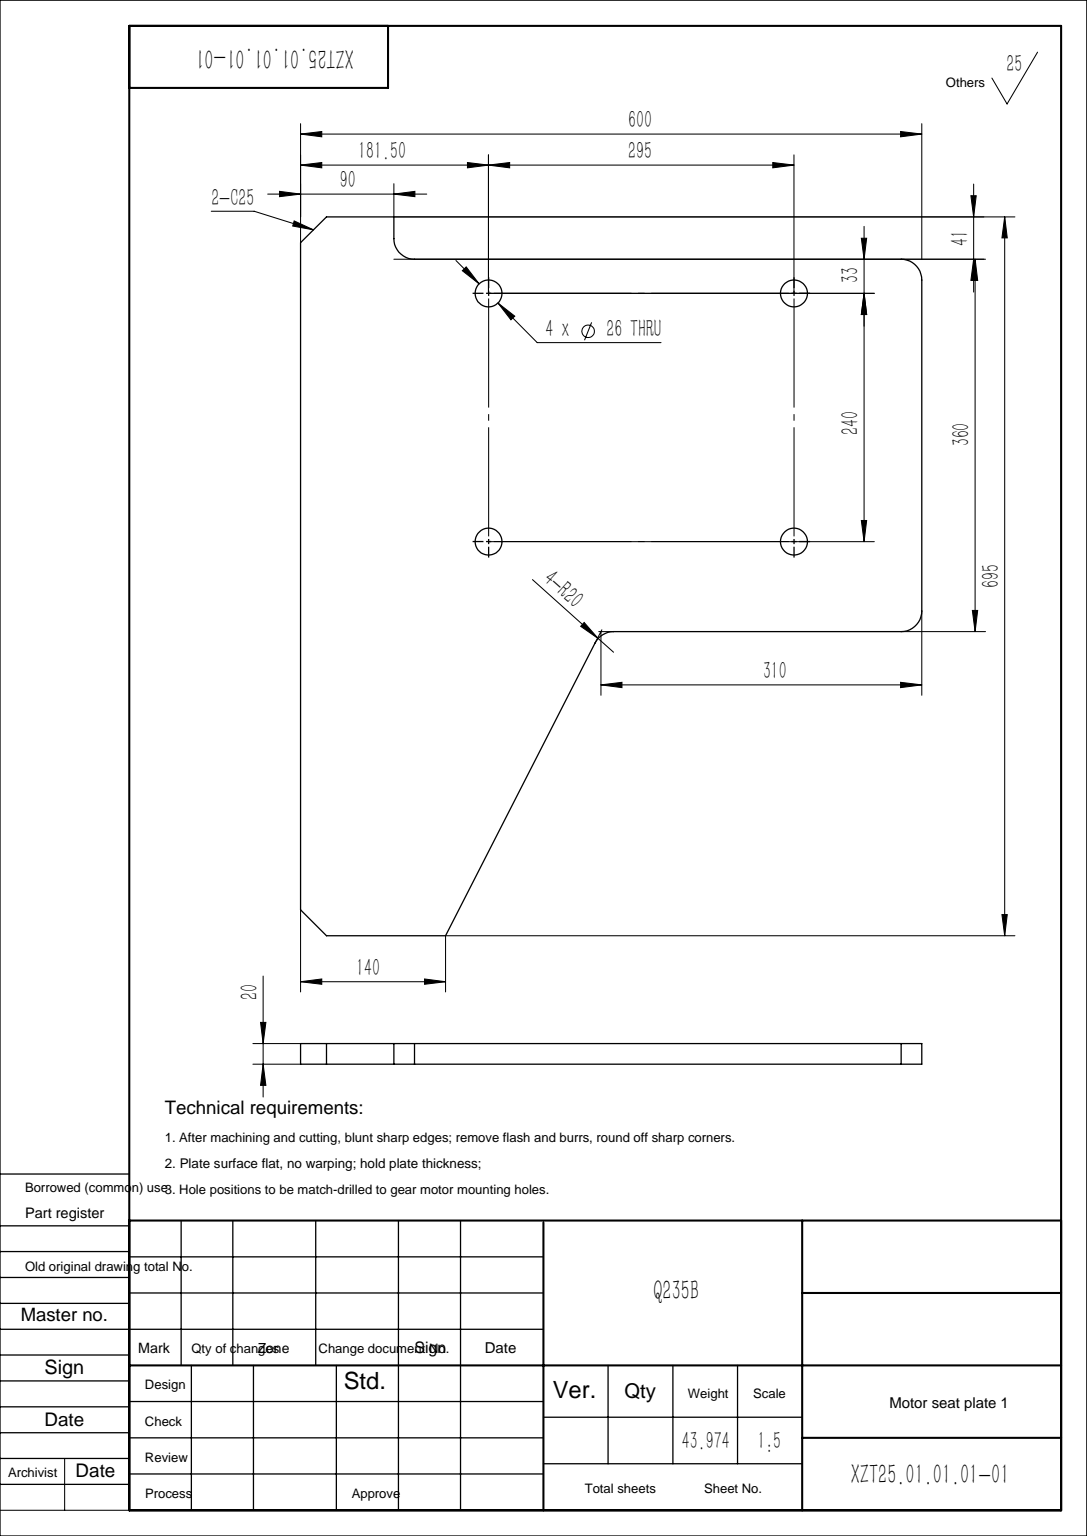
from build123d import *

# Parameters (mm, degrees)
BOSS_EXTRUDE1_DEPTH   = 10
CHAMFER1_SIZE         = 25
FILLET1_R             = 20
F_26_DIAMETER_HOLE1_D = 26


with BuildPart() as part:
    # Sketch1 → Boss-Extrude1 (new, symmetric)
    with BuildSketch(Plane.XY):
        Polygon((0, 0), (0, 695), (90, 695), (90, 654), (600, 654), (600, 294), (290, 294), (140, 0), align=None)
    extrude(amount=BOSS_EXTRUDE1_DEPTH, both=True)

    # Chamfer1
    chamfer1_edges = [part.edges().sort_by_distance(p)[0] for p in [
        (0, 0, 0),
        (0, 695, 0),
    ]]
    chamfer(chamfer1_edges, length=CHAMFER1_SIZE)

    # Fillet1
    fillet1_edges = [part.edges().sort_by_distance(p)[0] for p in [
        (90, 654, 0),
        (600, 654, 0),
        (600, 294, 0),
        (290, 294, 0),
    ]]
    fillet(fillet1_edges, radius=FILLET1_R)

    # Ø26 Diameter Hole1 (through all)
    with Locations(Plane.XY.offset(10)):
        with Locations((181.5, 621), (476.5, 621), (476.5, 381), (181.5, 381)):
            Hole(F_26_DIAMETER_HOLE1_D / 2)


solid = part.part
